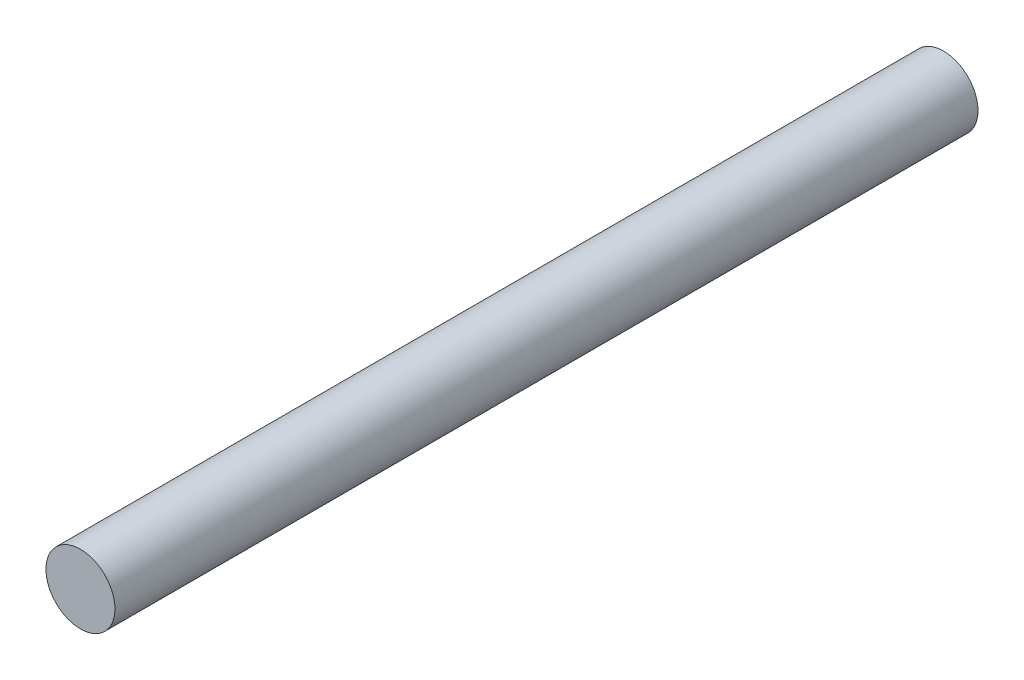
SolidWorks part; units mm, degrees
ref_plane "Front Plane" through (0, 0, 0) normal (0, 0, 1) x (1, 0, 0)
ref_plane "Top Plane" through (0, 0, 0) normal (0, 1, 0) x (1, 0, 0)
ref_plane "Right Plane" through (0, 0, 0) normal (1, 0, 0) x (0, 0, -1)
sketch "Sketch1" plane through (0, 0, 0) normal (0, 0, 1) x (1, 0, 0)
  circle A0 centre (0, 0) radius 8
  dimension "D1" = 16
extrude "Boss-Extrude1" add sketch "Sketch1" along normal blind 200
cosmetic thread "Cosmetic Thread1" parameters "D2"=15
